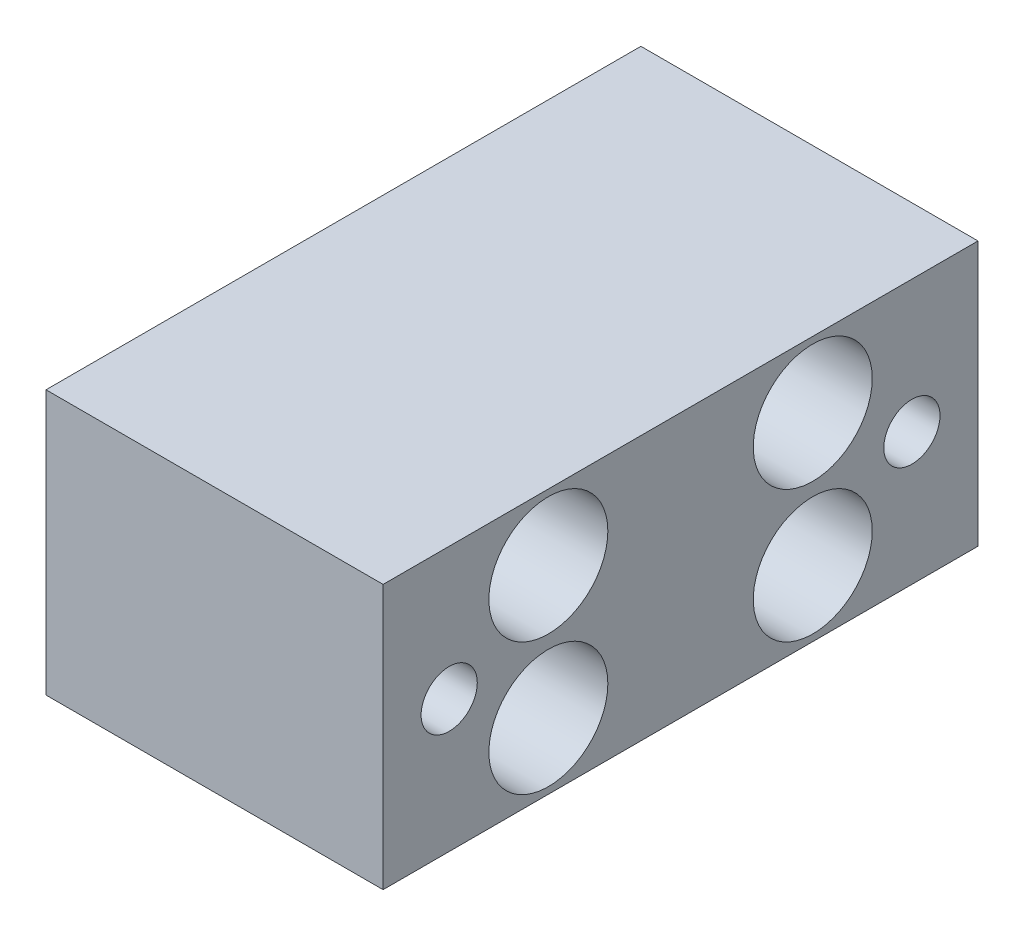
from build123d import *

# Parameters (mm, degrees)
SKETCH_1_W                = 90
SKETCH_1_H                = 40
EXTRUDE_1_DEPTH           = 51
HOLE_WIZARD_1_D           = 11
HOLE_WIZARD_1_CBORE_D     = 18
HOLE_WIZARD_1_CBORE_DEPTH = 40
HOLE_WIZARD_M10_1_D       = 8.5
HOLE_WIZARD_M10_1_DEPTH   = 24.5
HOLE_WIZARD_M10_1_TIP     = 2.553657631


with BuildPart() as part:
    # 草图1 → 凸台-拉伸1 (new body)
    with BuildSketch(Plane(origin=(0, 0, 0), x_dir=(0, 0, -1), z_dir=(1, 0, 0))):
        Rectangle(SKETCH_1_W, SKETCH_1_H)
    extrude(amount=EXTRUDE_1_DEPTH)

    # 打孔尺寸(%根据)内六角圆柱头螺钉的类型1 (through all)
    with Locations(Plane(origin=(51, 0, 0), x_dir=(0, 0, -1), z_dir=(1, 0, 0))):
        with Locations((-20, 10), (20, 10), (-20, -10), (20, -10)):
            CounterBoreHole(HOLE_WIZARD_1_D / 2, HOLE_WIZARD_1_CBORE_D / 2, HOLE_WIZARD_1_CBORE_DEPTH)

    # M10 螺纹孔1
    with Locations(Plane(origin=(51, 0, 0), x_dir=(0, 0, -1), z_dir=(1, 0, 0))):
        with Locations((-35, 0), (35, 0)):
            Hole(HOLE_WIZARD_M10_1_D / 2, depth=HOLE_WIZARD_M10_1_DEPTH)
            with Locations((0, 0, -(HOLE_WIZARD_M10_1_DEPTH + HOLE_WIZARD_M10_1_TIP / 2))):  # 118° drill point
                Cone(0, HOLE_WIZARD_M10_1_D / 2, HOLE_WIZARD_M10_1_TIP, mode=Mode.SUBTRACT)


solid = part.part
